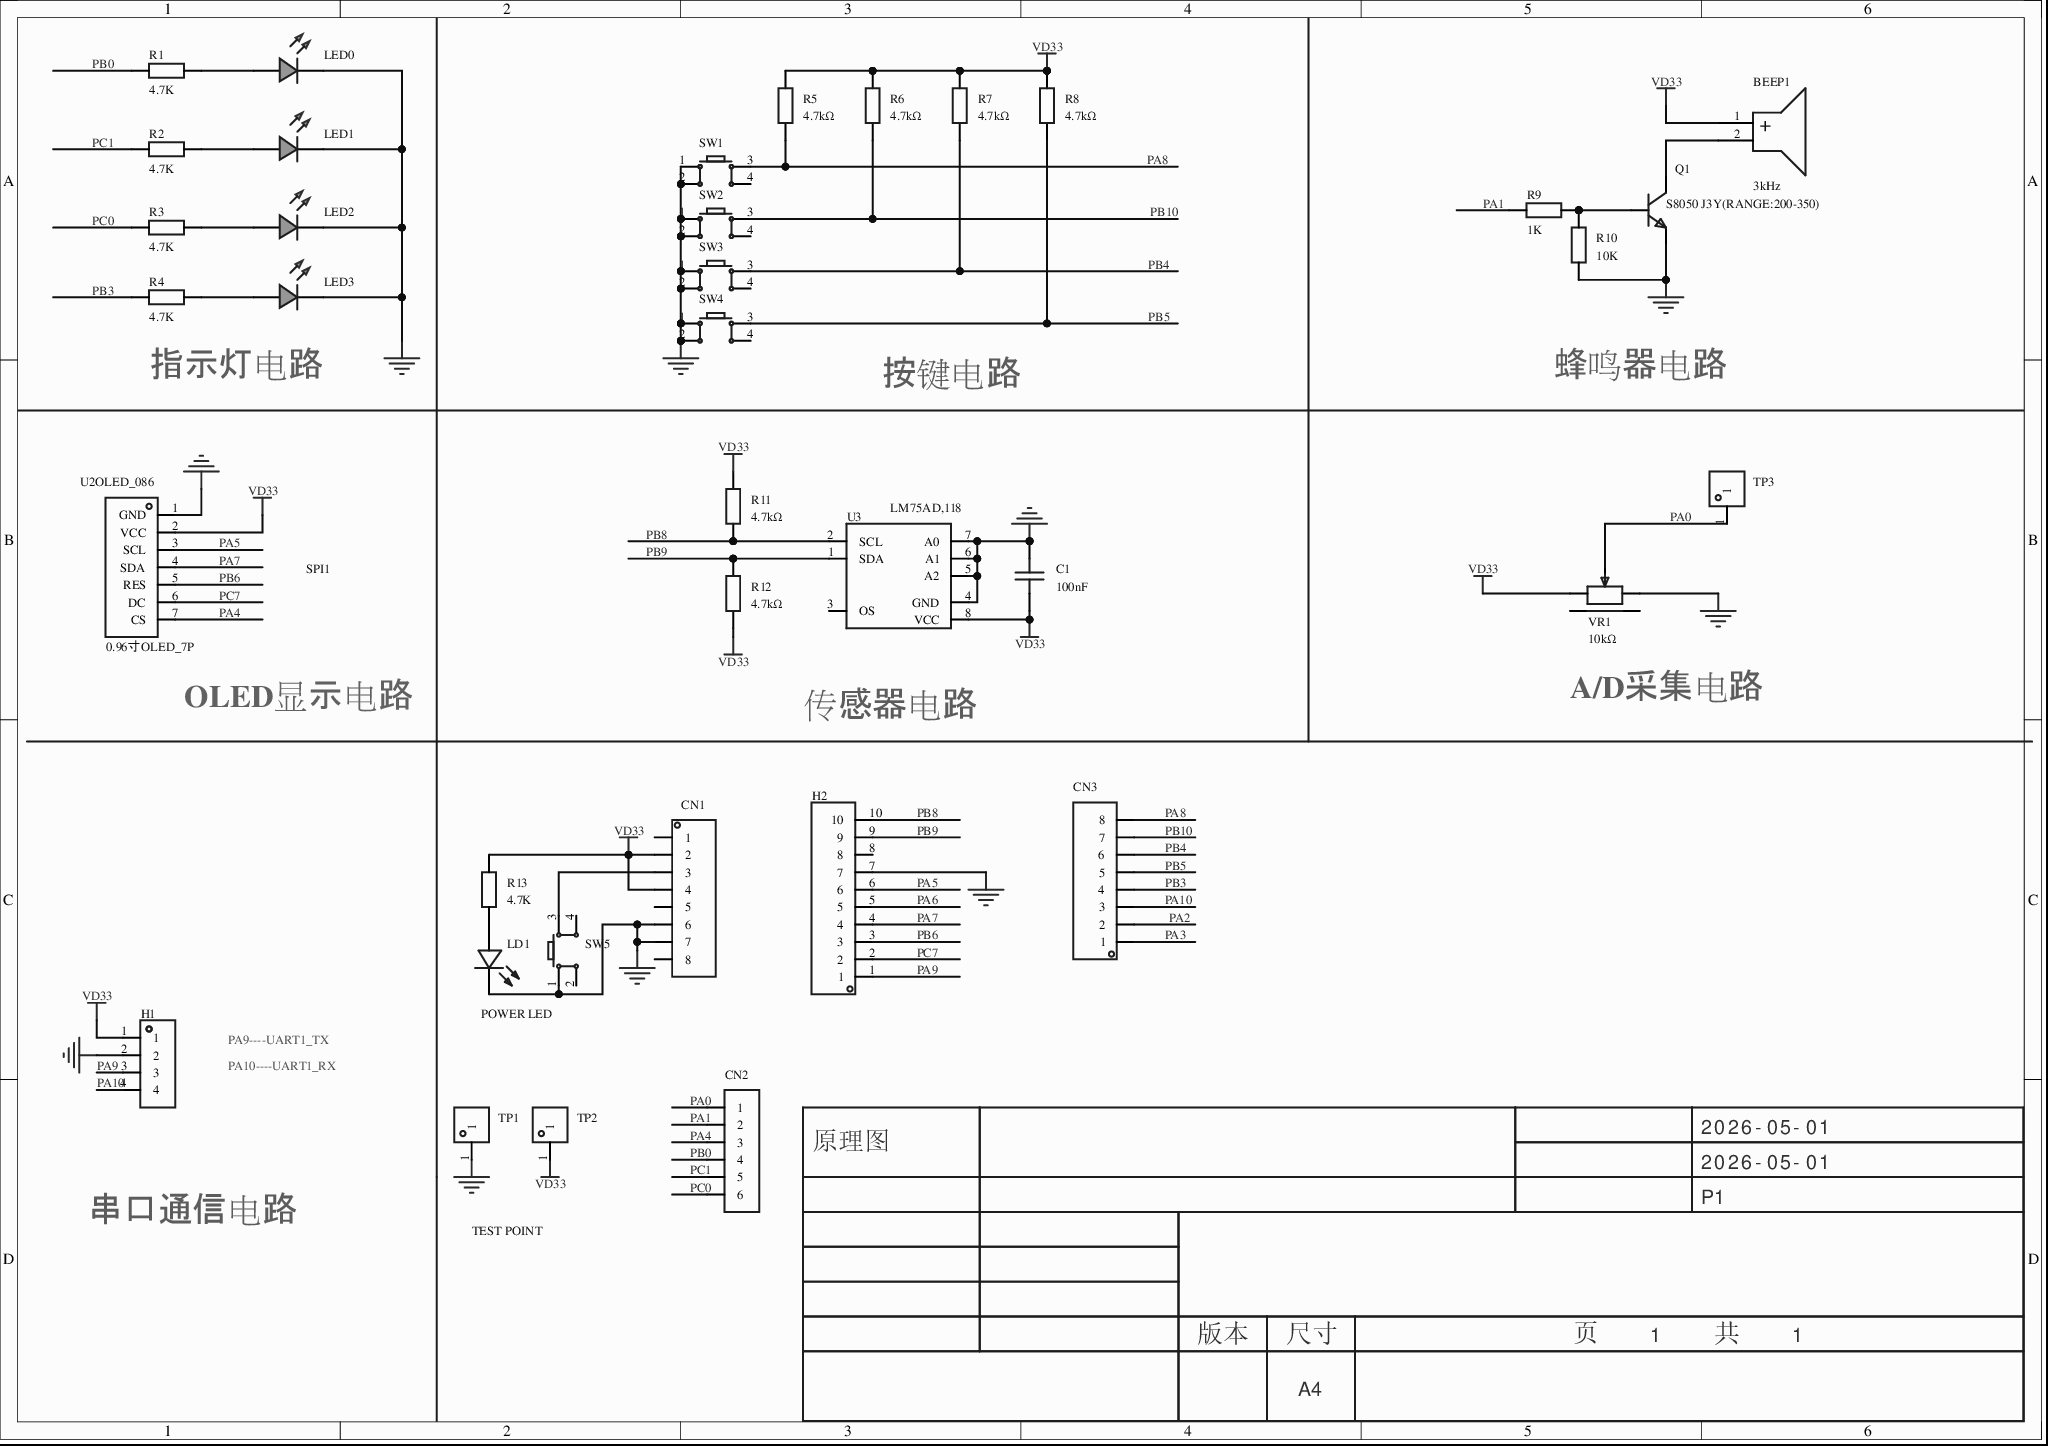
[diagram p0: MISC51904-3.schdoc]
# Altium project MISC51904-2.PrjPcb
1 sheet, 37 parts. Net scope: global (net labels, ports and power ports of the same name join across sheets).
Board file: MISC51904.pcbdoc

## Sheet MISC51904-3.schdoc
size 297 x 209 mm; Version: V1.0; @Project Name: MISC51904; @Update Date: 2026-05-01; @Create Date: 2026-05-01; @Board Name: MISC51904; @Create Time: 15:12:01; @Page Count: 1; @Page No: 1; @Schematic Name: MISC51904; @Update Time: 15:12:01; Size: A4

### Parts
BEEP1  3kHz  [BUZ-TH_BD9.0-P5.00-D0.6-FD]
C1  100nF  [C0805]
CN1  (no value)  [HDR-TH_8P-P2.54-V-M]
CN2  (no value)  [HDR-TH_6P-P2.54-V-M-1]
CN3  (no value)  [HDR-TH_8P-P2.54-V-M]
H1  (no value)  [HDR-TH_4P-P2.54-V-F]
H2  (no value)  [HDR-TH_10P-P2.54-V-M-1]
LD1  NCD0805R1  [LED0805-RD]  (value not drawn)
LED0  (no value)  [LED_0805]
LED1  (no value)  [LED_0805]
LED2  (no value)  [LED_0805]
LED3  (no value)  [LED_0805]
Q1  S8050 J3Y(RANGE:200-350)  [SOT-23-3_L3.0-W1.7-P0.95-LS2.9-BR]
R1  4.7K  [R0805]
R2  4.7K  [R0805]
R3  4.7K  [R0805]
R4  4.7K  [R0805]
R5  4.7kΩ  [R0805]
R6  4.7kΩ  [R0805]
R7  4.7kΩ  [R0805]
R8  4.7kΩ  [R0805]
R9  1K  [R0603]
R10  10K  [R0603]
R11  4.7kΩ  [R0805]
R12  4.7kΩ  [R0805]
R13  4.7K  [R0603]
SW1  (no value)  [Key_SMD_4.2x3.2x2.5]
SW2  (no value)  [Key_SMD_4.2x3.2x2.5]
SW3  (no value)  [Key_SMD_4.2x3.2x2.5]
SW4  (no value)  [Key_SMD_4.2x3.2x2.5]
SW5  (no value)  [Key_SMD_4.2x3.2x2.5]
TP1  TP-红色测试点  [TESTPOINT-TH_BD3.2]  (value not drawn)
TP2  TP-红色测试点  [TESTPOINT-TH_BD3.2]  (value not drawn)
TP3  TP-红色测试点  [TESTPOINT-TH_BD3.2]  (value not drawn)
U2OLED_086  0.96寸OLED_7P  [OLED-TH_HS96L01W4S03]
U3  LM75AD,118  [SOIC-8_L5.0-W4.0-P1.27-LS6.0-BL]
VR1  10kΩ  [RES-ADJ-TH_RK09K1130AJ3]

### Nets
GND: C1.2 CN1.6 CN1.7 H1.2 H2.7 LD1.1(-) LED0.1(C) LED1.1(C) LED2.1(C) LED3.1(C) Q1.2(E) R10.1 SW1.1 SW1.2 SW2.1 SW2.2 SW3.1 SW3.2 SW4.1 SW4.2 SW5.1 TP1.1 U2OLED_086.1(GND) U3.4(GND) U3.5(A2) U3.6(A1) U3.7(A0) VR1.1
VD33: BEEP1.1(+) C1.1 CN1.2 CN1.4 H1.1 R5.2 R6.2 R7.2 R8.2 R11.2 R12.1 R13.2 TP2.1 U2OLED_086.2(VCC) U3.8(VCC) VR1.3
PA0: CN2.1 TP3.1 VR1.2
PA1: CN2.2 R9.2
PA2: CN3.2
PA3: CN3.1
PA4: CN2.3 U2OLED_086.7(CS)
PA5: H2.6 U2OLED_086.3(SCL)
PA6: H2.5
PA7: H2.4 U2OLED_086.4(SDA)
PA8: CN3.8 R5.1 SW1.3
PA9: H1.3 H2.1
PA10: CN3.3 H1.4
PB0: CN2.4 R1.1
PB3: CN3.4 R4.1
PB4: CN3.6 R7.1 SW3.3
PB5: CN3.5 R8.1 SW4.3
PB6: H2.3 U2OLED_086.5(RES)
PB8: H2.10 R11.1 U3.2(SCL)
PB9: H2.9 R12.2 U3.1(SDA)
PB10: CN3.7 R6.1 SW2.3
PC0: CN2.6 R3.1
PC1: CN2.5 R2.1
PC7: H2.2 U2OLED_086.6(DC)
NetBEEP1_2: BEEP1.2(-) Q1.3(C)
NetCN1_3: CN1.3 SW5.3
NetLD1_2: LD1.2(+) R13.1
NetLED0_2: LED0.2(A) R1.2
NetLED1_2: LED1.2(A) R2.2
NetLED2_2: LED2.2(A) R3.2
NetLED3_2: LED3.2(A) R4.2
NetQ1_1: Q1.1(B) R9.1 R10.2

Not connected (* = marked no-connect by the designer): CN1 1* 5* 8*; H2 8*; SW1 4*; SW2 4*; SW3 4*; SW4 4*; SW5 2* 4*; U3 3(OS)*; VR1 4* 5*

### Notes on the sheet
- 指示灯电路
- 按键电路
- 蜂鸣器电路
- SPI1
- (near U2OLED_086) OLED显示电路
- 传感器电路
- (near VR1) A/D采集电路
- PA9----UART1_TX
- POWER LED
- PA10----UART1_RX
- 串口通信电路
- TEST POINT
- 2026-05-01
- 原理图
- P1
- 版本
- 尺寸
- A4
- 页    1    共    1

### Library data of the parts
BEEP1 = HNB09A03: 驱动方式:有源(内含驱动线路);构造类型:电磁式;频率:3kHz;声压(SPL):85dB;; Manufacturer: 华能; AddInBom: yes; ModelId: 13273335caac486e928bafb4d9fdf12d0819f05c4eef4c71ace90d822a990e87; ModelName: BUZ-TH_D9.0-H5.5-P5.0; ModelTransform: 354.33,354.33,0,90,0,0,-0.005,0,-177.165; Voltage - Supply: 1.5V~4.5V; Current Consumption: 30mA; Sound Pressure Level(SPL): 85dB; Symbol: HNB09A03; Device: HNB09A03; LCSC Part Name: 电磁式有源一体蜂鸣器HNB09A03; SupplierPart: C96102; ManufacturerPart: HNB09A03; Supplier Footprint: 插件,D=9mm; JLCPCB Part Class: Extended Part; Datasheet: https://item.szlcsc.com/datasheet/HNB09A03/97306.html; Supplier: LCSC; ConvertToPcb: yes; FootprintName: BUZ-TH_BD9.0-P5.00-D0.6-FD; Driver Circuitry: 有源(内含驱动线路); Technology: 电磁式; Value: 3kHz; Diameter(φD): 9mm; Length: -; Width: -; Height: 5.5mm; Operating Temperature: -20℃~+70℃
C1 = CC0805KRX7R9BB104: 容值:100nF;精度:±10%;额定电压:50V;温度系数:X7R;; Manufacturer: YAGEO(国巨); AddInBom: yes; ModelId: 1ba041120af144c991958decab20d2410819f05c4eef4c71ace90d822a990e87; ModelName: C0805_L2.0-W1.3-H1.3; ModelTransform: 78.74,51.181,0,0,0,0,0,0.0005,0; Tolerance: ±10%; Voltage Rating: 50V; Temperature Coefficient: X7R; Symbol: CC0805KRX7R9BB104; Device: CC0805KRX7R9BB104; LCSC Part Name: 100nF ±10% 50V; SupplierPart: C49678; ManufacturerPart: CC0805KRX7R9BB104; Supplier Footprint: 0805; JLCPCB Part Class: Basic Part; Datasheet: https://item.szlcsc.com/datasheet/CC0805KRX7R9BB104/50686.html; Supplier: LCSC; ConvertToPcb: yes; FootprintName: C0805; Value: 100nF
CN1 = HDR-M_2.54_1x8P: Symbol: Header-Male-2.54_1x8; ConvertToPcb: yes; ModelId: f5b96e27511e49e38545e53df23202020819f05c4eef4c71ace90d822a990e87; ModelTransform: 807.87244,98.425,0,0,0,0,0,0,-118.11; Device: HDR-M_2.54_1x8P; AddInBom: yes; SupplierPart: C124381; Supplier Footprint: 插件; FootprintName: HDR-TH_8P-P2.54-V-M; ModelName: HDR-TH_8P-P2.54-V-M
CN2 = HDR-M_2.54_1x6P: Symbol: Header-Male-2.54_1x6; ConvertToPcb: yes; ModelId: 60739dffc9b04830a286435b0fefbd4a0819f05c4eef4c71ace90d822a990e87; ModelName: HDR2.54-M-LI-1X6P; ModelTransform: 599.999,100,0,0,0,0,0,0,-118.11; Device: HDR-M_2.54_1x6P; AddInBom: yes; SupplierPart: C37208; Supplier Footprint: 插件; FootprintName: HDR-TH_6P-P2.54-V-M-1
CN3 = HDR-M_2.54_1x8P: Symbol: Header-Male-2.54_1x8; 3D Model: f5b96e27511e49e38545e53df23202020819f05c4eef4c71ace90d822a990e87; 3D Model Transform: 807.87244,98.425,0,0,0,0,0,0,-118.11; ConvertToPcb: yes; Device: HDR-M_2.54_1x8P; Supplier Part: C124381; Supplier Footprint: 插件; AddInBom: yes; FootprintName: HDR-TH_8P-P2.54-V-M; ModelName: HDR-TH_8P-P2.54-V-M
H1 = HDR-F_2.54_1x4P: Symbol: 2.54-1*4P母; ConvertToPcb: yes; ModelId: d187812051054f85879fcaa51a310d8e0819f05c4eef4c71ace90d822a990e87; ModelTransform: 419.6842,98.464,0,0,0,0,0,0,-118.11; Device: HDR-F_2.54_1x4P; AddInBom: yes; SupplierPart: C2718488; Supplier Footprint: 插件; FootprintName: HDR-TH_4P-P2.54-V-F; ModelName: HDR-TH_4P-P2.54-V-F
H2 = HDR-M_2.54_1x10P: Symbol: Header-Male-2.54_1x10; 3D Model: 10f3d1cea59e4bb4ba116af9f09c2b9b0819f05c4eef4c71ace90d822a990e87; 3D Model Transform: 999.99796,100,0,0,0,0,0,0,-118.11; ConvertToPcb: yes; ModelName: HDR2.54-M-LI-1X10P; Device: HDR-M_2.54_1x10P; Supplier Part: C57369; Supplier Footprint: 插件; AddInBom: yes; FootprintName: HDR-TH_10P-P2.54-V-M-1
LD1 = NCD0805R1: 灯头类型:-;发光颜色:红色;正向压降(Vf):1.6V~2.6V;功率:65mW;正向电流:25mA;波长:615nm~630nm;二极管配置:独立二极管;透镜颜色:-;色温:-;发光强度:195mcd;发光角度:130°;载带方式:-;工作温度:-30℃~+85℃;; Manufacturer: 国星光电; Symbol: FC-2012HRK-620D; AddInBom: yes; ModelId: b1c5ed7a4f6e46d3bc6f6cc7c20f3fea0819f05c4eef4c71ace90d822a990e87; ModelTransform: 79.527,49.2125,0,0,0,0,0,0,0; Illumination Color: 红色; Power(Watts): 65mW; Forward Current: 25mA; Peak Wavelength: 630nm; Diode Configuration: 独立二极管; Luminous Intensity: 195mcd; Viewing Angle: 130°; Device: NCD0805R1; LCSC Part Name: 片式发光二极管; SupplierPart: C84256; ManufacturerPart: NCD0805R1; Supplier Footprint: 0805; JLCPCB Part Class: Basic Part; Datasheet: https://item.szlcsc.com/datasheet/NCD0805R1/85425.html; Supplier: LCSC; ConvertToPcb: yes; FootprintName: LED0805-RD; ModelName: LED0805-RD; Lamp Holder Type: -; Voltage - Forward(Vf): 1.6V~2.6V; Wavelength - Dominant: 615nm~630nm; Lens Color: -; Color Temperature: -; Mounting Style: -; Operating Temperature: -30℃~+85℃
LED0-LED3 = LED_0805-G: Symbol: LED_G_OLD; Convert to PCB: yes; 3D Model: 381ae4d721d6485eaad9d0ca067812b50819f05c4eef4c71ace90d822a990e87; 3D Model Transform: 63.9,39.8,31.9,0,0,0,0,0,0; ModelName: LED-0805_G; Device: LED_0805-G; Add into BOM: yes; Supplier Footprint: 0805; FootprintName: LED_0805
Q1 = S8050 J3Y(RANGE:200-350): 晶体管类型:NPN;集电极电流(Ic):500mA;集射极击穿电压(Vceo):25V;耗散功率(Pd):300mW;直流电流增益(hFE):200@500mA,1V;; Manufacturer: CJ(江苏长电/长晶); Symbol: S8050_C2146; AddInBom: yes; ModelId: 89cb27a44ab2466697082bb9fd73a7d00819f05c4eef4c71ace90d822a990e87; ModelName: SOT-23-3L_L2.9-W1.6-H1.1-LS2.8-P0.95; ModelTransform: 114.173,110.236,0,90,0,0,0,0,0; type: NPN; Current - Collector(Ic): 500mA; Collector - Emitter Voltage VCEO: 25V; Pd - Power Dissipation: 300mW; Transition frequency(fT): 150MHz; Current - Collector Cutoff: 100nA; Vce Saturation(VCE(sat)): 600mV@500mA,50mA; Emitter-Base Voltage(Vebo): 5V; Number: 1个NPN; Device: S8050 J3Y(RANGE:200-350); LCSC Part Name: H档(200-350) NPN 电流:0.5A 电压:25V; SupplierPart: C2146; ManufacturerPart: S8050 J3Y(RANGE:200-350); Supplier Footprint: SOT-23; JLCPCB Part Class: Basic Part; Datasheet: https://item.szlcsc.com/datasheet/S8050%2520J3Y(RANGE%253A200-350)/2503.html; Supplier: LCSC; ConvertToPcb: yes; FootprintName: SOT-23-3_L3.0-W1.7-P0.95-LS2.9-BR; DC Current Gain: 200@500mA,1V; Operating Temperature: -55℃~+150℃
R1-R4 = Res_0805: Symbol: 电阻; 3D Model: 37a81e68749a4138bd2dfa6897b24b850819f05c4eef4c71ace90d822a990e87; 3D Model Transform: 78.74,51.181,0,0,0,0,0,-0.0005,0; ConvertToPcb: yes; ModelName: R0805_L2.0-W1.3-H0.6; Device: Res_0805; Supplier Footprint: 0805; Value: 4.7K; AddInBom: yes; FootprintName: R0805
R5-R8 R11 R12 = 0805W8F4701T5E: 电阻类型:厚膜电阻;阻值:4.7kΩ;精度:±1%;功率:125mW;最大工作电压:150V;温度系数:±100ppm/℃;; Manufacturer: UNI-ROYAL(厚声); AddInBom: yes; ModelId: 37a81e68749a4138bd2dfa6897b24b850819f05c4eef4c71ace90d822a990e87; ModelName: R0805_L2.0-W1.3-H0.6; ModelTransform: 78.74,51.181,0,0,0,0,0,-0.0005,0; Tolerance: ±1%; Power(Watts): 125mW; Overload Voltage (Max): 150V; Symbol: 0805W8F4701T5E; Device: 0805W8F4701T5E; LCSC Part Name: 4.7kΩ ±1% 125mW 厚膜电阻; SupplierPart: C17673; ManufacturerPart: 0805W8F4701T5E; Supplier Footprint: 0805; JLCPCB Part Class: Basic Part; Datasheet: https://atta.szlcsc.com/upload/public/pdf/source/20200306/C422600_1E6D84923E4A46A82E41ADD87F860B5C.pdf; Supplier: LCSC; ConvertToPcb: yes; FootprintName: R0805; Type: 厚膜电阻; Value: 4.7kΩ; Temperature Coefficient: ±100ppm/℃; Operating Temperature Range: -55℃~+155℃
R9 R10 = Res_0603: Symbol: 电阻; ConvertToPcb: yes; ModelId: fc143cca1e79419f9cd78b61e9279f080819f05c4eef4c71ace90d822a990e87; ModelTransform: 31.8897,63.7794,0,90,0,0,0,0,0; Device: Res_0603; AddInBom: yes; Supplier Footprint: 0603; FootprintName: R0603; ModelName: R0603
  R9: Value: 1K
  R10: Value: 10K
R13 = Res_0603: Symbol: 电阻; 3D Model: fc143cca1e79419f9cd78b61e9279f080819f05c4eef4c71ace90d822a990e87; 3D Model Transform: 31.8897,63.7794,0,90,0,0,0,0,0; ConvertToPcb: yes; Device: Res_0603; Supplier Footprint: 0603; Value: 4.7K; AddInBom: yes; FootprintName: R0603; ModelName: R0603
SW1-SW5 = Key_SMD_4.2x3.2x2.5: Symbol: 轻触按键; 3D Model: 38f4e5ae1c0a49d7a4c1f95a650cdbea0819f05c4eef4c71ace90d822a990e87; 3D Model Transform: 184.97,125.98,98.82,0,0,0,0,0,0; ConvertToPcb: yes; ModelName: KEY-SMD_4P-L4.2-W3.2-H2.5-LS4.6-P2.2; Device: Key_SMD_4.2x3.2x2.5; Supplier Footprint: SMD; AddInBom: yes; FootprintName: Key_SMD_4.2x3.2x2.5
TP1-TP3 = TP-红色测试点: AddInBom: yes; ModelId: 6bb19dcb8ff8413ea73fe7a5b79be1e30819f05c4eef4c71ace90d822a990e87; ModelTransform: 125.984,125.84132,0,0,0,0,0,0,-125.984; Symbol: TP-红色测试点; Device: TP-红色测试点; LCSC Part Name: TP-红色测试点; SupplierPart: C9900007423; ManufacturerPart: TP-红色测试点; Supplier Footprint: TESTPOINT-TH_BD-2P-P2.00; JLCPCB Part Class: Extended Part; Supplier: LCSC; ConvertToPcb: yes; FootprintName: TESTPOINT-TH_BD3.2; ModelName: TESTPOINT-TH_BD3.2
U2OLED_086 = HS96L01W4S03: 尺寸(inch):0.96;像素分辨率:128x64;; Manufacturer: HS(汉昇); AddInBom: yes; ModelId: 7927fe0e3c8842749d8ccfcaf6d2f4920819f05c4eef4c71ace90d822a990e87; ModelTransform: 1074.801,1094.486,0,0,0,0,0,-488.188,-157.48; Dot Pixels: 128x64; Type of Drive: 无源(PMOLED); Display Range: 21.74x10.86mm; Display Color: 白色; Luminance: 100cd/m2; Quiescent Current: 5uA; Symbol: HS96L01W4S03; Device: HS96L01W4S03; Manufacturer Part: 0.96寸OLED_7P; LCSC Part Name: 0.96寸 白光 128x64像素分辨率; SupplierPart: C5139758; Supplier Footprint: -; JLCPCB Part Class: Extended Part; Datasheet: https://item.szlcsc.com/datasheet/HS96L01W4S03/5751920.html; Supplier: LCSC; ConvertToPcb: yes; FootprintName: OLED-TH_HS96L01W4S03; ModelName: OLED-TH_HS96L01W4S03; Size: 0.96; Operating Temperature: -40℃~+80℃
U3 = LM75AD,118: 检测温度:-55℃~+125℃;精度:±2℃;接口类型:I2C;; Manufacturer: NXP(恩智浦); AddInBom: yes; ModelId: 7abc64c95a1a4a04a4ef38f9097c870b0819f05c4eef4c71ace90d822a990e87; ModelTransform: 192.913,236.22,0,0,0,0,0,0,0; Tolerance: ±2℃; Voltage - Supply: 2.8V~5.5V; Interface: I2C; Temperature Conversion Time: 100ms; Temperature Resolution: 11bit; Symbol: LM75AD; Device: LM75AD,118; LCSC Part Name: 数字温度传感器和热监控器; SupplierPart: C7963; ManufacturerPart: LM75AD,118; Supplier Footprint: SOIC-8; JLCPCB Part Class: Extended Part; Datasheet: https://www.nxp.com.cn/docs/en/data-sheet/LM75A.pdf; Supplier: LCSC; ConvertToPcb: yes; FootprintName: SOIC-8_L5.0-W4.0-P1.27-LS6.0-BL; ModelName: SOIC-8_L5.0-W4.0-P1.27-LS6.0-BL; Detection Temperature Range: -55℃~+125℃; Standby Current: -; Operating Temperature: -
VR1 = RK09K1130AJ3: 阻值:10kΩ;精度:±20%;功率:50mW;; Manufacturer: ALPSALPINE(阿尔卑斯阿尔派); AddInBom: yes; ModelId: 8d12f93edd6740baa62f8427ef4030010819f05c4eef4c71ace90d822a990e87; ModelTransform: 394.36653,472.44004,0,0,0,0,0,95.277,-157.48; Tolerance: ±20%; Voltage Rating: 20V; Power(Watts): 50mW; Symbol: RK09K1130AJ3; Device: RK09K1130AJ3; LCSC Part Name: 10kΩ ±20%; SupplierPart: C388854; ManufacturerPart: RK09K1130AJ3; Supplier Footprint: 插件; JLCPCB Part Class: Extended Part; Datasheet: https://item.szlcsc.com/datasheet/RK09K1130AJ3/364162.html; Supplier: LCSC; ConvertToPcb: yes; FootprintName: RES-ADJ-TH_RK09K1130AJ3; ModelName: RES-ADJ-TH_RK09K1130AJ3; Value: 10kΩ; Number of Turns: -